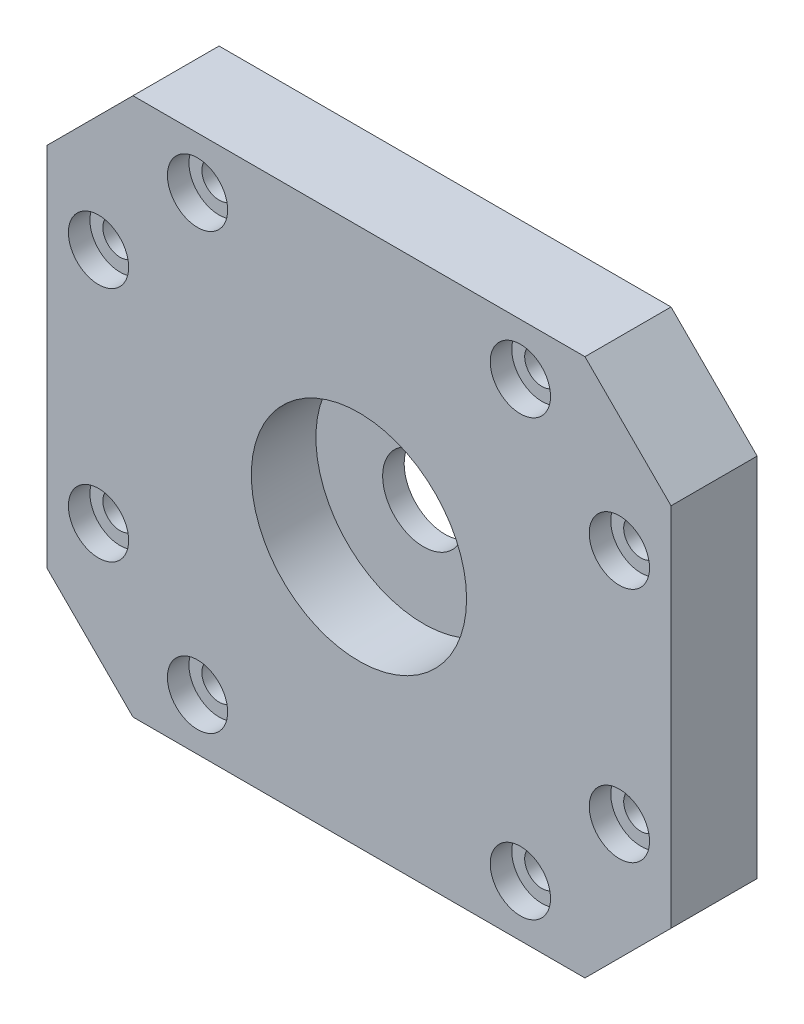
SolidWorks part; units mm, degrees
ref_plane "前视基准面" through (0, 0, 0) normal (0, 0, 1) x (1, 0, 0)
ref_plane "上视基准面" through (0, 0, 0) normal (0, 1, 0) x (1, 0, 0)
ref_plane "右视基准面" through (0, 0, 0) normal (1, 0, 0) x (0, 0, -1)
sketch "草图1" plane through (0, 0, 0) normal (0, 0, 1) x (1, 0, 0)
  line L1 (-72.5, -62.5) -> (72.5, -62.5)
  line L2 (-72.5, -62.5) -> (-72.5, 62.5)
  line L3 (-72.5, 62.5) -> (72.5, 62.5)
  line L4 (72.5, -62.5) -> (72.5, 62.5)
  line L5 (-72.5, -62.5) -> (72.5, 62.5) construction
  line L6 (-72.5, 62.5) -> (72.5, -62.5) construction
  point P0 (0, 0)
  dimension "D1" = 145
  dimension "D2" = 125
extrude "凸台-拉伸1" add sketch "草图1" along normal blind 20
chamfer "倒角1" distance 20 angle 45 4 edges at (-72.5, -62.5, 10) (72.5, -62.5, 10) (72.5, 62.5, 10) (-72.5, 62.5, 10)
sketch "草图2" plane through (0, 0, 20) normal (0, 0, 1) x (1, 0, 0)
  line L0 (52.5, 62.5) -> (-52.5, 62.5) construction
  line L1 (-72.5, 42.5) -> (-72.5, -42.5) construction
  line L2 (72.5, -42.5) -> (72.5, 42.5) construction
  line L3 (-52.5, -62.5) -> (52.5, -62.5) construction
  circle A0 centre (-37.5, 50.5) radius 7
  circle A1 centre (37.5, 50.5) radius 7
  circle A2 centre (-60.5, 27.5) radius 7
  circle A3 centre (-60.5, -27.5) radius 7
  circle A4 centre (-37.5, -50.5) radius 7
  circle A5 centre (37.5, -50.5) radius 7
  circle A6 centre (60.5, 27.5) radius 7
  circle A7 centre (60.5, -27.5) radius 7
extrude "切除-拉伸1" cut sketch "草图2" against normal blind 5
sketch "草图3" plane through (0, 0, 15) normal (0, 0, 1) x (1, 0, 0)
  circle A0 centre (-37.5, 50.5) radius 4
  circle A1 centre (-60.5, 27.5) radius 4
  circle A2 centre (-60.5, -27.5) radius 4
  circle A3 centre (-37.5, -50.5) radius 4
  circle A4 centre (37.5, 50.5) radius 4
  circle A5 centre (60.5, 27.5) radius 4
  circle A6 centre (60.5, -27.5) radius 4
  circle A7 centre (37.5, -50.5) radius 4
  dimension "D1" = 8
extrude "切除-拉伸2" cut sketch "草图3" against normal up to next
sketch "草图4" plane through (0, 0, 0) normal (0, 0, -1) x (-1, 0, 0)
  line L1 (19, 15.5) -> (-19, 15.5)
  line L2 (19, 15.5) -> (19, -15.5)
  line L3 (19, -15.5) -> (-19, -15.5)
  line L4 (-19, 15.5) -> (-19, -15.5)
  line L5 (19, 15.5) -> (-19, -15.5) construction
  line L6 (19, -15.5) -> (-19, 15.5) construction
  point P0 (0, 0)
  dimension "D1" = 31
  dimension "D2" = 38
extrude "切除-拉伸3" [suppressed] cut sketch "草图4" against normal blind 1.5
sketch "草图5" [suppressed] plane through (0, 0, 0) normal (0, 0, -1) x (-1, 0, 0)
  circle A0 centre (19, -15.5) radius 2.5
  circle A1 centre (-19, -15.5) radius 2.5
  circle A2 centre (-19, 15.5) radius 2.5
  circle A3 centre (19, 15.5) radius 2.5
  dimension "D1" = 5
extrude "切除-拉伸4" [suppressed] cut sketch "草图5" against normal blind 1.5
sketch "草图6" plane through (0, 0, 0) normal (0, 0, -1) x (-1, 0, 0)
  circle A0 centre (0, 0) radius 9.5
  dimension "D1" = 19
extrude "切除-拉伸5" cut sketch "草图6" against normal up to next
sketch "草图7" plane through (0, 0, 20) normal (0, 0, 1) x (1, 0, 0)
  circle A0 centre (0, 0) radius 25
  dimension "D1" = 50
extrude "切除-拉伸6" cut sketch "草图7" against normal blind 15
equation "\"D5@草图2\"=\"D4@草图2\""
equation "\"D6@草图2\"=\"D4@草图2\""
equation "\"D7@草图2\"=\"D2@草图2\""
equation "\"D8@草图2\"=\"D2@草图2\""
equation "\"D9@草图2\"=\"D2@草图2\""
equation "\"D3@草图2\"=\"D4@草图2\""
